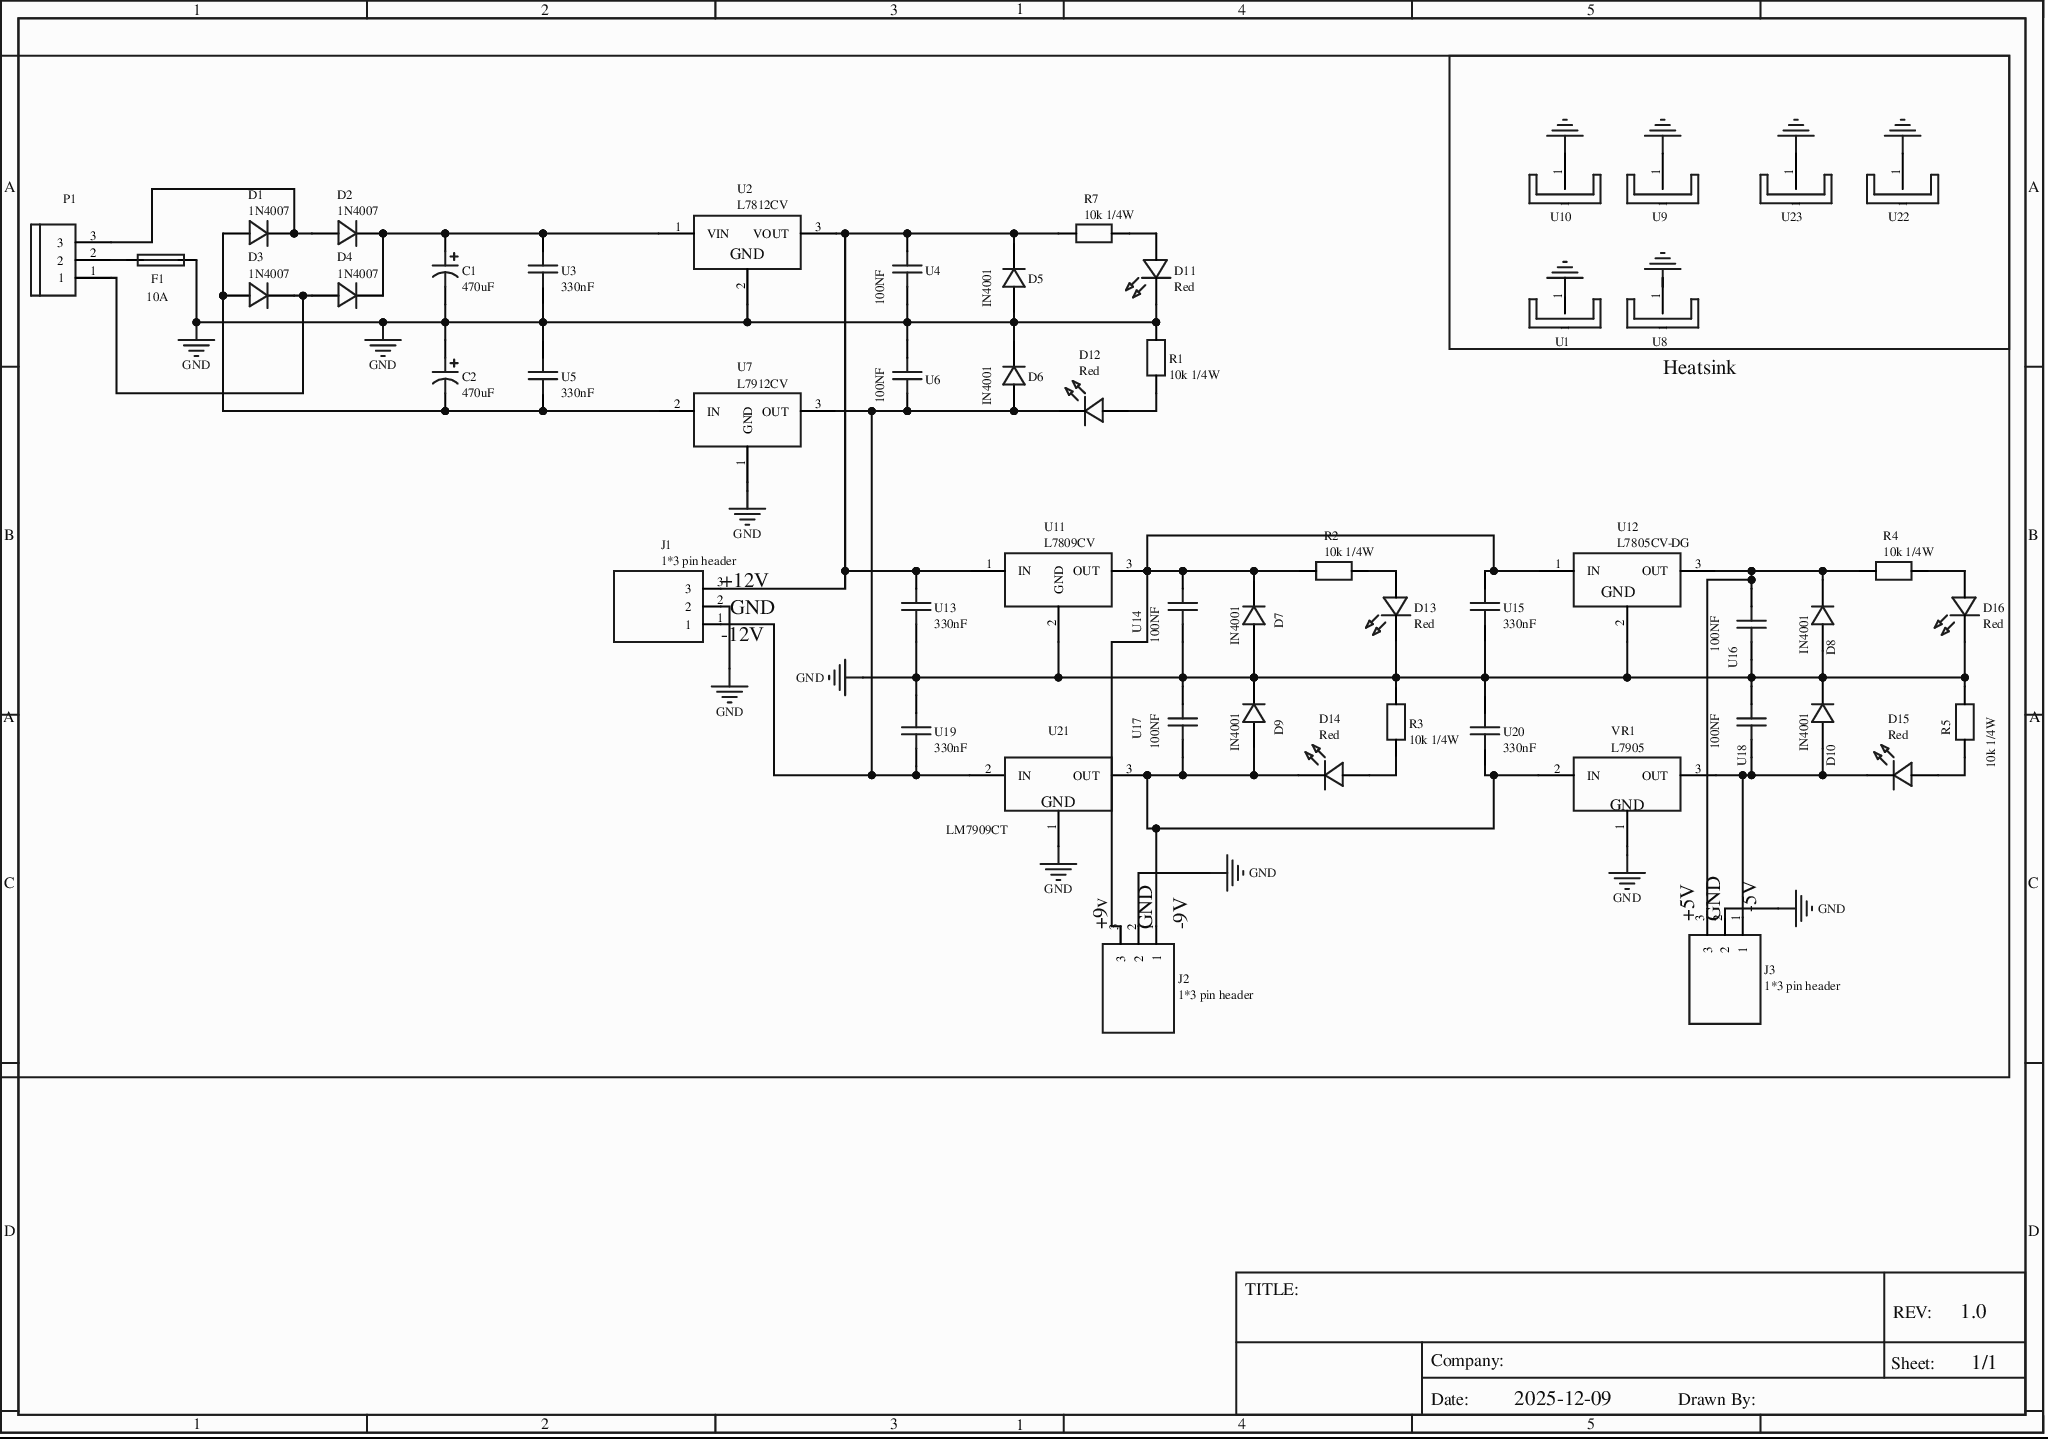
[diagram p0: MISC51935-3.schdoc]
# Altium project MISC51935-2.PrjPcb
1 sheet, 53 parts. Net scope: global (net labels, ports and power ports of the same name join across sheets).
Board file: MISC51935.pcbdoc

## Sheet MISC51935-3.schdoc
size 292 x 204 mm; Name: MISC51935; @Project Name: MISC51935; REV: 1.0; Date: 2025-12-09; Sheet: 1/1; spicePre: .

### Parts
C1  470uF  [CAP-TH_BD10.0-P5.00-D0.6-FD]
C2  470uF  [CAP-TH_BD10.0-P5.00-D0.6-FD]
D1  1N4007  [DO-41_BD2.4-L4.7-P8.70-D0.9-RD]
D2  1N4007  [DO-41_BD2.4-L4.7-P8.70-D0.9-RD]
D3  1N4007  [DO-41_BD2.4-L4.7-P8.70-D0.9-RD]
D4  1N4007  [DO-41_BD2.4-L4.7-P8.70-D0.9-RD]
D5  IN4001  [DO-41_BD2.4-L4.7-P8.70-D0.9-RD]
D6  IN4001  [DO-41_BD2.4-L4.7-P8.70-D0.9-RD]
D7  IN4001  [DO-41_BD2.4-L4.7-P8.70-D0.9-RD]
D8  IN4001  [DO-41_BD2.4-L4.7-P8.70-D0.9-RD]
D9  IN4001  [DO-41_BD2.4-L4.7-P8.70-D0.9-RD]
D10  IN4001  [DO-41_BD2.4-L4.7-P8.70-D0.9-RD]
D11  Red  [发光二极管]
D12  Red  [发光二极管]
D13  Red  [发光二极管]
D14  Red  [发光二极管]
D15  Red  [发光二极管]
D16  Red  [发光二极管]
F1  10A  [FUSE-SMD_5-20MM]
J1  1*3 pin header  [1*3排针]
J2  1*3 pin header  [1*3排针]
J3  1*3 pin header  [1*3排针]
P1  WJ500V-5.08-3P  [CONN-TH_3P-P5.00_WJ500V-5.08-3P]  (value not drawn)
R1  10k 1/4W  [10K直插电阻 PCB封装]
R2  10k 1/4W  [10K直插电阻 PCB封装]
R3  10k 1/4W  [10K直插电阻 PCB封装]
R4  10k 1/4W  [10K直插电阻 PCB封装]
R5  10k 1/4W  [10K直插电阻 PCB封装]
R7  10k 1/4W  [10K直插电阻 PCB封装]
U1  15*10.5*21  [SINK-TH_L15.0-W10.5-H21.0]  (value not drawn)
U2  L7812CV  [TO-220-3_L10.0-W4.5-P2.54-T]
U3  330nF  [CAP-TH_L10.0-W4.0-P7.50-D0.6-1]
U4  100NF  [CAP-TH_L5.0-W2.5-P5.00-D1.0]
U5  330nF  [CAP-TH_L10.0-W4.0-P7.50-D0.6-1]
U6  100NF  [CAP-TH_L5.0-W2.5-P5.00-D1.0]
U7  L7912CV  [TO-220-3_L10.0-W4.5-P2.54-L]
U8  15*10.5*21  [SINK-TH_L15.0-W10.5-H21.0]  (value not drawn)
U9  15*10.5*21  [SINK-TH_L15.0-W10.5-H21.0]  (value not drawn)
U10  15*10.5*21  [SINK-TH_L15.0-W10.5-H21.0]  (value not drawn)
U11  L7809CV  [TO-220-3_L10.0-W4.5-P2.54-L]
U12  L7805CV-DG  [TO-220-3_L10.0-W4.5-P2.54-L]
U13  330nF  [CAP-TH_L10.0-W4.0-P7.50-D0.6-1]
U14  100NF  [CAP-TH_L5.0-W2.5-P5.00-D1.0]
U15  330nF  [CAP-TH_L10.0-W4.0-P7.50-D0.6-1]
U16  100NF  [CAP-TH_L5.0-W2.5-P5.00-D1.0]
U17  100NF  [CAP-TH_L5.0-W2.5-P5.00-D1.0]
U18  100NF  [CAP-TH_L5.0-W2.5-P5.00-D1.0]
U19  330nF  [CAP-TH_L10.0-W4.0-P7.50-D0.6-1]
U20  330nF  [CAP-TH_L10.0-W4.0-P7.50-D0.6-1]
U21  LM7909CT  [TO-220-3_L10.0-W4.5-P2.54-L]
U22  15*10.5*21  [SINK-TH_L15.0-W10.5-H21.0]  (value not drawn)
U23  15*10.5*21  [SINK-TH_L15.0-W10.5-H21.0]  (value not drawn)
VR1  L7905  [TO-220-3_L10.0-W4.5-P2.54-L]

### Nets
GND: C1.2 C2.1 D5.2 D6.1 D7.2 D8.2 D9.1 D10.1 D11.2 D13.2 D16.2 F1.2 J1.2 J2.2 J3.2 R1.2 R3.2 R5.2 U1.1 U2.2(GND) U3.1 U4.2 U5.2 U6.1 U7.1(GND) U8.1 U9.1 U10.1 U11.2(GND) U12.2(GND) U13.1 U14.2 U15.1 U16.2 U17.1 U18.1 U19.2 U20.2 U21.1(GND) U22.1 U23.1 VR1.1(GND)
NetC1_1: C1.1 D2.1(K) D4.1(K) U2.1(VIN) U3.2
NetC2_2: C2.2 D1.2(A) D3.2(A) U5.1 U7.2(IN)
NetD1_1: D1.1(K) D2.2(A) P1.3
NetD3_1: D3.1(K) D4.2(A) P1.1
NetD5_1: D5.1 J1.3 R7.1 U2.3(VOUT) U4.1 U11.1(IN) U13.2
NetD6_2: D6.2 D12.2 J1.1 U6.2 U7.3(OUT) U19.1 U21.2(IN)
NetD7_1: D7.1 J2.3 R2.1 U11.3(OUT) U12.1(IN) U14.1 U15.2
NetD8_1: D8.1 J3.3 R4.1 U12.3(OUT) U16.1
NetD9_2: D9.2 D14.2 J2.1 U17.2 U20.1 U21.3(OUT) VR1.2(IN)
NetD10_2: D10.2 D15.2 J3.1 U18.2 VR1.3(OUT)
NetD11_1: D11.1 R7.2
NetD12_1: D12.1 R1.1
NetD13_1: D13.1 R2.2
NetD14_1: D14.1 R3.1
NetD15_1: D15.1 R5.1
NetD16_1: D16.1 R4.2
NetF1_1: F1.1 P1.2

### Notes on the sheet
- (near U8) Heatsink
- (near J1) -12V
- (near J1) +12V
- (near J1) GND
- (near J2) +9v
- (near J2) GND
- (near J2) -9V
- (near J3) +5V
- (near J3) GND
- (near J3) -5V
- 1
- 2
- 3
- 4
- 5
- A
- B
- C
- D
- TITLE:
- Company:
- Sheet:
- REV:
- 1.0
- 1/1
- Date:
- 2025-12-09
- Drawn By:

### Library data of the parts
C1 = 470uF: Manufacturer: KNSCHA(科尼盛); Manufacturer Part: 01EC1266; nameAlias: Value; Contributor: LCSC; Convert to PCB: yes; UniqueId: ggeb4693cfd16d534cd; Origin Footprint: CAP-TH_BD10.0-P5.00-D0.6-FD; Device: 470uF; Symbol: 470uF; Supplier: LCSC; Supplier Part: C2831772; JLCPCB Part Class: Extended Part; spicePre: C; spiceSymbolName: 01EC1266; Add into BOM: yes; FootprintName: CAP-TH_BD10.0-P5.00-D0.6-FD
C2 = 470uF: Manufacturer: KNSCHA(科尼盛); Manufacturer Part: 01EC1266; nameAlias: Value; Contributor: LCSC; Convert to PCB: yes; UniqueId: ggea2c5d49bc5dde298; Origin Footprint: CAP-TH_BD10.0-P5.00-D0.6-FD; Device: 470uF; Symbol: 470uF; Supplier: LCSC; Supplier Part: C2831772; JLCPCB Part Class: Extended Part; spicePre: C; spiceSymbolName: 01EC1266; Add into BOM: yes; FootprintName: CAP-TH_BD10.0-P5.00-D0.6-FD
D1 = 1N4007: Manufacturer: ST(先科); Convert to PCB: yes; UniqueId: gge6eb2f7ba7a12821c; Origin Footprint: DO-41_BD2.4-L4.7-P8.70-D0.9-RD; Device: 1N4007; Symbol: 1N4007; Supplier: LCSC; Manufacturer Part: 1N4007; Supplier Part: C106903; JLCPCB Part Class: Extended Part; spicePre: D; spiceSymbolName: 1N4007; Add into BOM: yes; FootprintName: DO-41_BD2.4-L4.7-P8.70-D0.9-RD
D2 = 1N4007: Manufacturer: ST(先科); Convert to PCB: yes; UniqueId: ggecca08e5caf06c018; Origin Footprint: DO-41_BD2.4-L4.7-P8.70-D0.9-RD; Device: 1N4007; Symbol: 1N4007; Supplier: LCSC; Manufacturer Part: 1N4007; Supplier Part: C106903; JLCPCB Part Class: Extended Part; spicePre: D; spiceSymbolName: 1N4007; Add into BOM: yes; FootprintName: DO-41_BD2.4-L4.7-P8.70-D0.9-RD
D3 = 1N4007: Manufacturer: ST(先科); Convert to PCB: yes; UniqueId: gge81689f1d3303caec; Origin Footprint: DO-41_BD2.4-L4.7-P8.70-D0.9-RD; Device: 1N4007; Symbol: 1N4007; Supplier: LCSC; Manufacturer Part: 1N4007; Supplier Part: C106903; JLCPCB Part Class: Extended Part; spicePre: D; spiceSymbolName: 1N4007; Add into BOM: yes; FootprintName: DO-41_BD2.4-L4.7-P8.70-D0.9-RD
D4 = 1N4007: Manufacturer: ST(先科); Convert to PCB: yes; UniqueId: gge6a4368da87585c93; Origin Footprint: DO-41_BD2.4-L4.7-P8.70-D0.9-RD; Device: 1N4007; Symbol: 1N4007; Supplier: LCSC; Manufacturer Part: 1N4007; Supplier Part: C106903; JLCPCB Part Class: Extended Part; spicePre: D; spiceSymbolName: 1N4007; Add into BOM: yes; FootprintName: DO-41_BD2.4-L4.7-P8.70-D0.9-RD
D5 = IN4001: Manufacturer: DIOFIT(對餘科技); Manufacturer Part: 1N4004; Contributor: djwao_ybk; Convert to PCB: yes; UniqueId: ggeaa27cf4c2f614704; Origin Footprint: DO-41_BD2.4-L4.7-P8.70-D0.9-RD; Device: IN4001; Symbol: IN4001; Supplier Part: C169151; Supplier: LCSC; JLCPCB Part Class: Extended Part; spicePre: D; spiceSymbolName: 1N4004-C169151; Add into BOM: yes; FootprintName: DO-41_BD2.4-L4.7-P8.70-D0.9-RD
D6 = IN4001: Manufacturer: DIOFIT(對餘科技); Manufacturer Part: 1N4004; Contributor: djwao_ybk; Convert to PCB: yes; UniqueId: gge0b466d7a0d9696a1; Origin Footprint: DO-41_BD2.4-L4.7-P8.70-D0.9-RD; Device: IN4001; Symbol: IN4001; Supplier Part: C169151; Supplier: LCSC; JLCPCB Part Class: Extended Part; spicePre: D; spiceSymbolName: 1N4004-C169151; Add into BOM: yes; FootprintName: DO-41_BD2.4-L4.7-P8.70-D0.9-RD
D7 = IN4001: Manufacturer: DIOFIT(對餘科技); Manufacturer Part: 1N4004; Contributor: djwao_ybk; Convert to PCB: yes; UniqueId: gge61ba849a9213f6b6; Origin Footprint: DO-41_BD2.4-L4.7-P8.70-D0.9-RD; Device: IN4001; Symbol: IN4001; Supplier Part: C169151; Supplier: LCSC; JLCPCB Part Class: Extended Part; spicePre: D; spiceSymbolName: 1N4004-C169151; Add into BOM: yes; FootprintName: DO-41_BD2.4-L4.7-P8.70-D0.9-RD
D8 = IN4001: Manufacturer: DIOFIT(對餘科技); Manufacturer Part: 1N4004; Contributor: djwao_ybk; Convert to PCB: yes; UniqueId: gged726a396729c3148; Origin Footprint: DO-41_BD2.4-L4.7-P8.70-D0.9-RD; Device: IN4001; Symbol: IN4001; Supplier Part: C169151; Supplier: LCSC; JLCPCB Part Class: Extended Part; spicePre: D; spiceSymbolName: 1N4004-C169151; Add into BOM: yes; FootprintName: DO-41_BD2.4-L4.7-P8.70-D0.9-RD
D9 = IN4001: Manufacturer: DIOFIT(對餘科技); Manufacturer Part: 1N4004; Contributor: djwao_ybk; Convert to PCB: yes; UniqueId: ggeff0c81595de38f51; Origin Footprint: DO-41_BD2.4-L4.7-P8.70-D0.9-RD; Device: IN4001; Symbol: IN4001; Supplier Part: C169151; Supplier: LCSC; JLCPCB Part Class: Extended Part; spicePre: D; spiceSymbolName: 1N4004-C169151; Add into BOM: yes; FootprintName: DO-41_BD2.4-L4.7-P8.70-D0.9-RD
D10 = IN4001: Manufacturer: DIOFIT(對餘科技); Manufacturer Part: 1N4004; Contributor: djwao_ybk; Convert to PCB: yes; UniqueId: gge260e63abbc5bbcdd; Origin Footprint: DO-41_BD2.4-L4.7-P8.70-D0.9-RD; Device: IN4001; Symbol: IN4001; Supplier Part: C169151; Supplier: LCSC; JLCPCB Part Class: Extended Part; spicePre: D; spiceSymbolName: 1N4004-C169151; Add into BOM: yes; FootprintName: DO-41_BD2.4-L4.7-P8.70-D0.9-RD
D11 = Red: Manufacturer: EVERLIGHT(台湾亿光); Manufacturer Part: 204-10SDRD/S530-A3-L; Origin Footprint: LED; Contributor: PERSON_A; Convert to PCB: yes; UniqueId: gge4a025b23dd483e77; Device: Red; Symbol: Red; Supplier Part: C84774; Supplier: LCSC; spicePre: L; spiceSymbolName: LED-TH-3mm_R; Add into BOM: yes; FootprintName: LED
D12 = Red: Manufacturer: EVERLIGHT(台湾亿光); Manufacturer Part: 204-10SDRD/S530-A3-L; Origin Footprint: LED; Contributor: PERSON_A; Convert to PCB: yes; UniqueId: ggee5b6fafad02cb5e5; Device: Red; Symbol: Red; Supplier Part: C84774; Supplier: LCSC; spicePre: L; spiceSymbolName: LED-TH-3mm_R; Add into BOM: yes; FootprintName: LED
D13 = Red: Manufacturer: EVERLIGHT(台湾亿光); Manufacturer Part: 204-10SDRD/S530-A3-L; Origin Footprint: LED; Contributor: PERSON_A; Convert to PCB: yes; UniqueId: ggece11eae628bf0898; Device: Red; Symbol: Red; Supplier Part: C84774; Supplier: LCSC; spicePre: L; spiceSymbolName: LED-TH-3mm_R; Add into BOM: yes; FootprintName: LED
D14 = Red: Manufacturer: EVERLIGHT(台湾亿光); Manufacturer Part: 204-10SDRD/S530-A3-L; Origin Footprint: LED; Contributor: PERSON_A; Convert to PCB: yes; UniqueId: ggecfb83bff858ff60b; Device: Red; Symbol: Red; Supplier Part: C84774; Supplier: LCSC; spicePre: L; spiceSymbolName: LED-TH-3mm_R; Add into BOM: yes; FootprintName: LED
D15 = Red: Manufacturer: EVERLIGHT(台湾亿光); Manufacturer Part: 204-10SDRD/S530-A3-L; Origin Footprint: LED; Contributor: PERSON_A; Convert to PCB: yes; UniqueId: gge5a0673a142bc4553; Device: Red; Symbol: Red; Supplier Part: C84774; Supplier: LCSC; spicePre: L; spiceSymbolName: LED-TH-3mm_R; Add into BOM: yes; FootprintName: LED
D16 = Red: Manufacturer: EVERLIGHT(台湾亿光); Manufacturer Part: 204-10SDRD/S530-A3-L; Origin Footprint: LED; Contributor: PERSON_A; Convert to PCB: yes; UniqueId: gge699199f951af46ee; Device: Red; Symbol: Red; Supplier Part: C84774; Supplier: LCSC; spicePre: L; spiceSymbolName: LED-TH-3mm_R; Add into BOM: yes; FootprintName: LED
F1 = 10A: Manufacturer Part: 5F.2500210000R1; Manufacturer: xcfuse(旭程); Contributor: 7ensen; Convert to PCB: yes; UniqueId: gge09f31a4987c8a883; Origin Footprint: FUSE-SMD_5-20MM; Device: 10A; Symbol: 10A; Supplier: LCSC; Supplier Part: C14518; JLCPCB Part Class: Extended Part; spicePre: F; spiceSymbolName: 2.5A 250V; Add into BOM: yes; FootprintName: FUSE-SMD_5-20MM
J1 = 1*3排针: Contributor: wthh; Package Display: No; Convert to PCB: yes; UniqueId: gge20fb3c7b60a69496; Origin Footprint: 1*3 pin header; Device: 1*3 pin header; Symbol: 1*3 pin header; spicePre: J; spiceSymbolName: 1*3 pin header; Add into BOM: yes; FootprintName: 1*3 pin header
J2 = 1*3排针: Contributor: wthh; Convert to PCB: yes; UniqueId: gge8ea73ede18738d88; Origin Footprint: 1*3 pin header; Device: 1*3 pin header; Symbol: 1*3 pin header; spicePre: J; spiceSymbolName: 1*3 pin header; Add into BOM: yes; FootprintName: 1*3 pin header
J3 = 1*3排针: Contributor: wthh; Convert to PCB: yes; UniqueId: gge924f517a26d7a59d; Origin Footprint: 1*3 pin header; Device: 1*3 pin header; Symbol: 1*3 pin header; spicePre: J; spiceSymbolName: 1*3 pin header; Add into BOM: yes; FootprintName: 1*3 pin header
P1 = WJ500V-5.08-3P: Manufacturer: KANGNEX(康奈克斯电气); Add into BOM: yes; Pitch: 5.08mm; Structure: 1x3P; Number of PINs Per Row: 3; Current Rating (Max): 18A; Voltage Rating (Max): 250V; Wire Gauge - AWG: 14~30; Wire Gauge - mm2: 2.5; Contributor: Ruici_OPA; UniqueId: ggec39ee3c861a7b382; Origin Footprint: CONN-TH_3P-P5.00_WJ500V-5.08-3P; Device: WJ500V-5.08-3P; Symbol: WJ500V-5.08-3P; LCSC Part Name: 5.08mm 1x3P 排数:1 每排P数:3 直插 可拼接; Supplier Part: C72334; Manufacturer Part: WJ500V-5.08-3P; Supplier Footprint: 插件,P=5.08mm; JLCPCB Part Class: Extended Part; Datasheet: https://atta.szlcsc.com/upload/public/pdf/source/20191225/C72334_8A5EF831D67650233B6B1E3F2BC06274.pdf; Supplier: LCSC; Convert to PCB: yes; Number of Rows: 1; Mounting Style: Through-hole; Operating Temperature Range: -40℃~+105℃; Color: Green; Number of Pins: 3P; value: WJ500V-5.08-3P; spicePre: P; spiceSymbolName: WJ500V-5.08-3P; FootprintName: CONN-TH_3P-P5.00_WJ500V-5.08-3P
R1 = 10k 1/4W: Origin Footprint: 10K through-hole resistor PCB footprint; nameAlias: Value(Ω); Contributor: qinmaochang; Convert to PCB: yes; UniqueId: ggefc82c9929f8d1236; Device: 10k 1/4W; Symbol: 10k 1/4W; spicePre: R; spiceSymbolName: R_0603_EU; Add into BOM: yes; FootprintName: 10K through-hole resistor PCB footprint
R2 = 10k 1/4W: Origin Footprint: 10K through-hole resistor PCB footprint; nameAlias: Value(Ω); Contributor: qinmaochang; Convert to PCB: yes; UniqueId: gge0a3a1e48c0925dad; Device: 10k 1/4W; Symbol: 10k 1/4W; spicePre: R; spiceSymbolName: R_0603_EU; Add into BOM: yes; FootprintName: 10K through-hole resistor PCB footprint
R3 = 10k 1/4W: Origin Footprint: 10K through-hole resistor PCB footprint; nameAlias: Value(Ω); Contributor: qinmaochang; Convert to PCB: yes; UniqueId: gge83760e001ccf7397; Device: 10k 1/4W; Symbol: 10k 1/4W; spicePre: R; spiceSymbolName: R_0603_EU; Add into BOM: yes; FootprintName: 10K through-hole resistor PCB footprint
R4 = 10k 1/4W: Origin Footprint: 10K through-hole resistor PCB footprint; nameAlias: Value(Ω); Contributor: qinmaochang; Convert to PCB: yes; UniqueId: ggea3ff81bada2f421f; Device: 10k 1/4W; Symbol: 10k 1/4W; spicePre: R; spiceSymbolName: R_0603_EU; Add into BOM: yes; FootprintName: 10K through-hole resistor PCB footprint
R5 = 10k 1/4W: Origin Footprint: 10K through-hole resistor PCB footprint; nameAlias: Value(Ω); Contributor: qinmaochang; Convert to PCB: yes; UniqueId: ggece3a59315397d48d; Device: 10k 1/4W; Symbol: 10k 1/4W; spicePre: R; spiceSymbolName: R_0603_EU; Add into BOM: yes; FootprintName: 10K through-hole resistor PCB footprint
R7 = 10k 1/4W: Origin Footprint: 10K through-hole resistor PCB footprint; nameAlias: Value(Ω); Contributor: qinmaochang; Convert to PCB: yes; UniqueId: gge2def4a741ed9176a; Device: 10k 1/4W; Symbol: 10k 1/4W; spicePre: R; spiceSymbolName: R_0603_EU; Add into BOM: yes; FootprintName: 10K through-hole resistor PCB footprint
U1 = 15*10.5*21: Manufacturer: XSD(鑫顺达); Manufacturer Part: 15.5*10.5*21; Contributor: LCSC; Convert to PCB: yes; UniqueId: gge1bdc0ab44f99f92d; Origin Footprint: SINK-TH_L15.0-W10.5-H21.0; Device: 15*10.5*21; Symbol: 15*10.5*21; Supplier: LCSC; Supplier Part: C4649; JLCPCB Part Class: Extended Part; spicePre: U; spiceSymbolName: 15*10.5*21; Add into BOM: yes; FootprintName: SINK-TH_L15.0-W10.5-H21.0
U2 = L7812CV: Manufacturer: ST(意法半导体); Contributor: houminghui; Convert to PCB: yes; UniqueId: gge48f0ae2437312dae; Origin Footprint: TO-220-3_L10.0-W4.5-P2.54-T; Device: L7812CV; Symbol: L7812CV; Supplier: LCSC; Manufacturer Part: L7812CV; Supplier Part: C105651; JLCPCB Part Class: Extended Part; spicePre: U; spiceSymbolName: L7812CV; Add into BOM: yes; FootprintName: TO-220-3_L10.0-W4.5-P2.54-T
U3 = 330nF: Manufacturer: TDK; Manufacturer Part: B32520C1334J189; Contributor: lcsc; nameAlias: Value; Convert to PCB: yes; UniqueId: gge66797bcd97f4f6c2; Origin Footprint: CAP-TH_L10.0-W4.0-P7.50-D0.6-1; Device: 330nF; Symbol: 330nF; Supplier: LCSC; Supplier Part: C3767460; JLCPCB Part Class: Extended Part; spicePre: U; spiceSymbolName: B32520C1334J189; Add into BOM: yes; FootprintName: CAP-TH_L10.0-W4.0-P7.50-D0.6-1
U4 = 100NF: Manufacturer: null; Contributor: lcsc; Convert to PCB: yes; UniqueId: ggebac468049775df37; Origin Footprint: CAP-TH_L5.0-W2.5-P5.00-D1.0; Device: 100NF; Symbol: 100NF; Supplier: LCSC; Supplier Part: C9900015256; Manufacturer Part: 100nF; spicePre: U; spiceSymbolName: 100NF_C9900015256; Add into BOM: yes; FootprintName: CAP-TH_L5.0-W2.5-P5.00-D1.0
U5 = 330nF: Manufacturer: TDK; Manufacturer Part: B32520C1334J189; Contributor: lcsc; nameAlias: Value; Convert to PCB: yes; UniqueId: ggeadf583383e4d69d4; Origin Footprint: CAP-TH_L10.0-W4.0-P7.50-D0.6-1; Device: 330nF; Symbol: 330nF; Supplier: LCSC; Supplier Part: C3767460; JLCPCB Part Class: Extended Part; spicePre: U; spiceSymbolName: B32520C1334J189; Add into BOM: yes; FootprintName: CAP-TH_L10.0-W4.0-P7.50-D0.6-1
U6 = 100NF: Manufacturer: null; Contributor: lcsc; Convert to PCB: yes; UniqueId: gge124c013cfc851acc; Origin Footprint: CAP-TH_L5.0-W2.5-P5.00-D1.0; Device: 100NF; Symbol: 100NF; Supplier: LCSC; Supplier Part: C9900015256; Manufacturer Part: 100nF; spicePre: U; spiceSymbolName: 100NF_C9900015256; Add into BOM: yes; FootprintName: CAP-TH_L5.0-W2.5-P5.00-D1.0
U7 = L7912CV: Manufacturer: ST(意法半导体); Convert to PCB: yes; UniqueId: gge4ec783ed4741de1f; Origin Footprint: TO-220-3_L10.0-W4.5-P2.54-L; Device: L7912CV; Symbol: L7912CV; Supplier: LCSC; Manufacturer Part: L7912CV; Supplier Part: C111886; JLCPCB Part Class: Extended Part; spicePre: U; spiceSymbolName: L7912CV; Add into BOM: yes; FootprintName: TO-220-3_L10.0-W4.5-P2.54-L
U8 = 15*10.5*21: Manufacturer: XSD(鑫顺达); Manufacturer Part: 15.5*10.5*21; Contributor: LCSC; Convert to PCB: yes; UniqueId: gge484e3008dca2bfa8; Origin Footprint: SINK-TH_L15.0-W10.5-H21.0; Device: 15*10.5*21; Symbol: 15*10.5*21; Supplier: LCSC; Supplier Part: C4649; JLCPCB Part Class: Extended Part; spicePre: U; spiceSymbolName: 15*10.5*21; Add into BOM: yes; FootprintName: SINK-TH_L15.0-W10.5-H21.0
U9 = 15*10.5*21: Manufacturer: XSD(鑫顺达); Manufacturer Part: 15.5*10.5*21; Contributor: LCSC; Convert to PCB: yes; UniqueId: gge2dbbb3175ebf36d7; Origin Footprint: SINK-TH_L15.0-W10.5-H21.0; Device: 15*10.5*21; Symbol: 15*10.5*21; Supplier: LCSC; Supplier Part: C4649; JLCPCB Part Class: Extended Part; spicePre: U; spiceSymbolName: 15*10.5*21; Add into BOM: yes; FootprintName: SINK-TH_L15.0-W10.5-H21.0
U10 = 15*10.5*21: Manufacturer: XSD(鑫顺达); Manufacturer Part: 15.5*10.5*21; Contributor: LCSC; Convert to PCB: yes; UniqueId: ggec69de7c088414df5; Origin Footprint: SINK-TH_L15.0-W10.5-H21.0; Device: 15*10.5*21; Symbol: 15*10.5*21; Supplier: LCSC; Supplier Part: C4649; JLCPCB Part Class: Extended Part; spicePre: U; spiceSymbolName: 15*10.5*21; Add into BOM: yes; FootprintName: SINK-TH_L15.0-W10.5-H21.0
U11 = L7809CV: Manufacturer: ST(意法半导体); Contributor: hxytliu; Convert to PCB: yes; UniqueId: gge2fd166bdb6936536; Origin Footprint: TO-220-3_L10.0-W4.5-P2.54-L; Device: L7809CV; Symbol: L7809CV; Supplier: LCSC; Manufacturer Part: L7809CV; Supplier Part: C8091; JLCPCB Part Class: Extended Part; spicePre: U; spiceSymbolName: L7809CV; Add into BOM: yes; FootprintName: TO-220-3_L10.0-W4.5-P2.54-L
U12 = L7805CV-DG: Manufacturer: ST(意法半导体); Convert to PCB: yes; UniqueId: ggeb6112465b0588c80; Origin Footprint: TO-220-3_L10.0-W4.5-P2.54-L; Device: L7805CV-DG; Symbol: L7805CV-DG; Supplier: LCSC; Manufacturer Part: L7805CV-DG; Supplier Part: C3795; JLCPCB Part Class: Extended Part; spicePre: U; spiceSymbolName: L7805CV-DG; Add into BOM: yes; FootprintName: TO-220-3_L10.0-W4.5-P2.54-L
U13 = 330nF: Manufacturer: TDK; Manufacturer Part: B32520C1334J189; Contributor: lcsc; nameAlias: Value; Convert to PCB: yes; UniqueId: gge95e557ff5ab9d76b; Origin Footprint: CAP-TH_L10.0-W4.0-P7.50-D0.6-1; Device: 330nF; Symbol: 330nF; Supplier: LCSC; Supplier Part: C3767460; JLCPCB Part Class: Extended Part; spicePre: U; spiceSymbolName: B32520C1334J189; Add into BOM: yes; FootprintName: CAP-TH_L10.0-W4.0-P7.50-D0.6-1
U14 = 100NF: Manufacturer: null; Contributor: lcsc; Convert to PCB: yes; UniqueId: gge8791d75d94e1481b; Origin Footprint: CAP-TH_L5.0-W2.5-P5.00-D1.0; Device: 100NF; Symbol: 100NF; Supplier: LCSC; Supplier Part: C9900015256; Manufacturer Part: 100nF; spicePre: U; spiceSymbolName: 100NF_C9900015256; Add into BOM: yes; FootprintName: CAP-TH_L5.0-W2.5-P5.00-D1.0
U15 = 330nF: Manufacturer: TDK; Manufacturer Part: B32520C1334J189; Contributor: lcsc; nameAlias: Value; Convert to PCB: yes; UniqueId: gge28995c53ef78d865; Origin Footprint: CAP-TH_L10.0-W4.0-P7.50-D0.6-1; Device: 330nF; Symbol: 330nF; Supplier: LCSC; Supplier Part: C3767460; JLCPCB Part Class: Extended Part; spicePre: U; spiceSymbolName: B32520C1334J189; Add into BOM: yes; FootprintName: CAP-TH_L10.0-W4.0-P7.50-D0.6-1
U16 = 100NF: Manufacturer: null; Contributor: lcsc; Convert to PCB: yes; UniqueId: ggeca4d2b64b6ec8380; Origin Footprint: CAP-TH_L5.0-W2.5-P5.00-D1.0; Device: 100NF; Symbol: 100NF; Supplier: LCSC; Supplier Part: C9900015256; Manufacturer Part: 100nF; spicePre: U; spiceSymbolName: 100NF_C9900015256; Add into BOM: yes; FootprintName: CAP-TH_L5.0-W2.5-P5.00-D1.0
U17 = 100NF: Manufacturer: null; Contributor: lcsc; Convert to PCB: yes; UniqueId: gge1a5dee1823ef113a; Origin Footprint: CAP-TH_L5.0-W2.5-P5.00-D1.0; Device: 100NF; Symbol: 100NF; Supplier: LCSC; Supplier Part: C9900015256; Manufacturer Part: 100nF; spicePre: U; spiceSymbolName: 100NF_C9900015256; Add into BOM: yes; FootprintName: CAP-TH_L5.0-W2.5-P5.00-D1.0
U18 = 100NF: Manufacturer: null; Contributor: lcsc; Convert to PCB: yes; UniqueId: gge3b01714176430545; Origin Footprint: CAP-TH_L5.0-W2.5-P5.00-D1.0; Device: 100NF; Symbol: 100NF; Supplier: LCSC; Supplier Part: C9900015256; Manufacturer Part: 100nF; spicePre: U; spiceSymbolName: 100NF_C9900015256; Add into BOM: yes; FootprintName: CAP-TH_L5.0-W2.5-P5.00-D1.0
U19 = 330nF: Manufacturer: TDK; Manufacturer Part: B32520C1334J189; Contributor: lcsc; nameAlias: Value; Convert to PCB: yes; UniqueId: ggea4a6b0395ae03088; Origin Footprint: CAP-TH_L10.0-W4.0-P7.50-D0.6-1; Device: 330nF; Symbol: 330nF; Supplier: LCSC; Supplier Part: C3767460; JLCPCB Part Class: Extended Part; spicePre: U; spiceSymbolName: B32520C1334J189; Add into BOM: yes; FootprintName: CAP-TH_L10.0-W4.0-P7.50-D0.6-1
U20 = 330nF: Manufacturer: TDK; Manufacturer Part: B32520C1334J189; Contributor: lcsc; nameAlias: Value; Convert to PCB: yes; UniqueId: ggebbc2f931070973b7; Origin Footprint: CAP-TH_L10.0-W4.0-P7.50-D0.6-1; Device: 330nF; Symbol: 330nF; Supplier: LCSC; Supplier Part: C3767460; JLCPCB Part Class: Extended Part; spicePre: U; spiceSymbolName: B32520C1334J189; Add into BOM: yes; FootprintName: CAP-TH_L10.0-W4.0-P7.50-D0.6-1
U21 = LM7909CT: Manufacturer: ON Semicon; Contributor: yanjq; Convert to PCB: yes; UniqueId: gge2c27b242a2875aaf; Origin Footprint: TO-220-3_L10.0-W4.5-P2.54-L; Device: LM7909CT; Symbol: LM7909CT; Supplier: LCSC; Supplier Part: C133149; Manufacturer Part: LM7909CT; spicePre: U; spiceSymbolName: LM7909CT; Add into BOM: yes; FootprintName: TO-220-3_L10.0-W4.5-P2.54-L
U22 = 15*10.5*21: Manufacturer: XSD(鑫顺达); Manufacturer Part: 15.5*10.5*21; Contributor: LCSC; Convert to PCB: yes; UniqueId: ggeb94fd32bcc95872d; Origin Footprint: SINK-TH_L15.0-W10.5-H21.0; Device: 15*10.5*21; Symbol: 15*10.5*21; Supplier: LCSC; Supplier Part: C4649; JLCPCB Part Class: Extended Part; spicePre: U; spiceSymbolName: 15*10.5*21; Add into BOM: yes; FootprintName: SINK-TH_L15.0-W10.5-H21.0
U23 = 15*10.5*21: Manufacturer: XSD(鑫顺达); Manufacturer Part: 15.5*10.5*21; Contributor: LCSC; Convert to PCB: yes; UniqueId: ggebe87043ebfc5f98d; Origin Footprint: SINK-TH_L15.0-W10.5-H21.0; Device: 15*10.5*21; Symbol: 15*10.5*21; Supplier: LCSC; Supplier Part: C4649; JLCPCB Part Class: Extended Part; spicePre: U; spiceSymbolName: 15*10.5*21; Add into BOM: yes; FootprintName: SINK-TH_L15.0-W10.5-H21.0
VR1 = L7905: Contributor: h3348619677; Package Display: No; Convert to PCB: yes; UniqueId: gge8e857b1cff8fa7ed; Origin Footprint: TO-220-3_L10.0-W4.5-P2.54-L; Device: L7905; Symbol: L7905; spicePre: U; spiceSymbolName: to-220-3; Add into BOM: yes; FootprintName: TO-220-3_L10.0-W4.5-P2.54-L